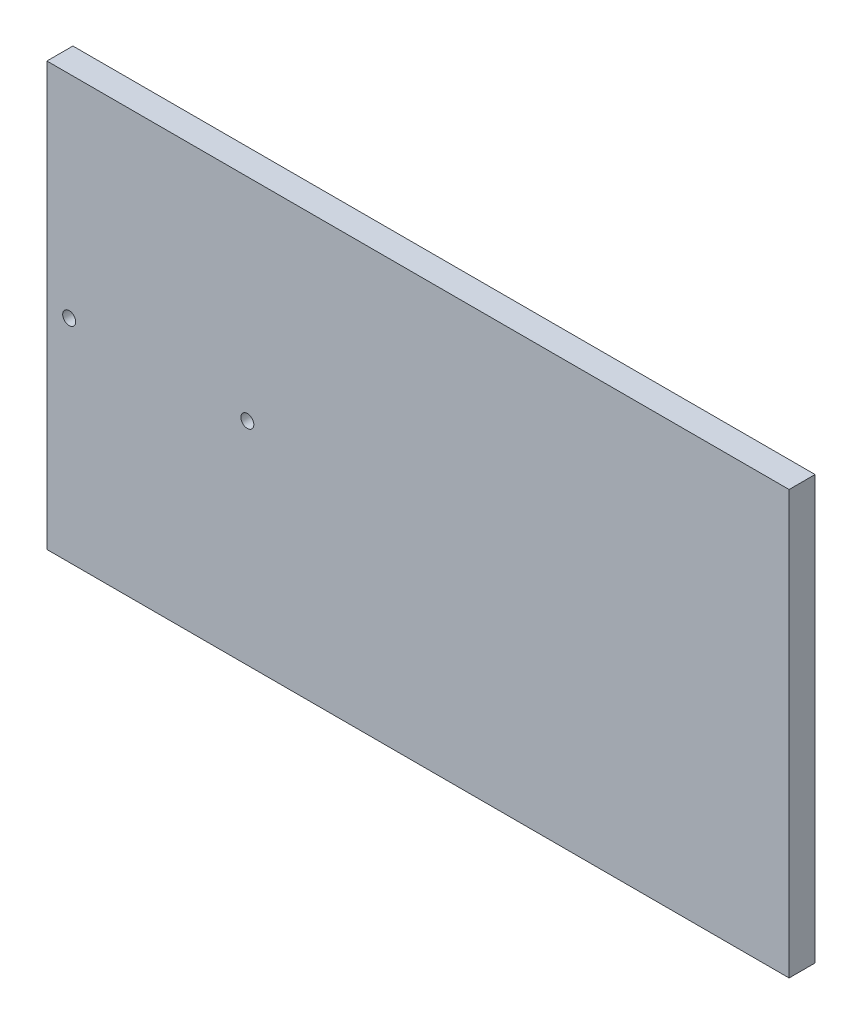
from build123d import *

# Parameters (mm, degrees)
SKETCH1_W           = 1000
SKETCH1_H           = 570
BOSS_EXTRUDE1_DEPTH = 35
M20_TAPPED_HOLE1_D  = 17.5


with BuildPart() as part:
    # Sketch1 → Boss-Extrude1 (new body)
    with BuildSketch(Plane.XY):
        with Locations((500, 285)):
            Rectangle(SKETCH1_W, SKETCH1_H)
    extrude(amount=BOSS_EXTRUDE1_DEPTH)

    # M20 Tapped Hole1 (through all)
    with Locations(Plane(origin=(30, 285, 35), x_dir=(1, 0, 0), z_dir=(0, 0, 1))):
        with Locations((0, 0), (240, 0)):
            Hole(M20_TAPPED_HOLE1_D / 2)


solid = part.part
